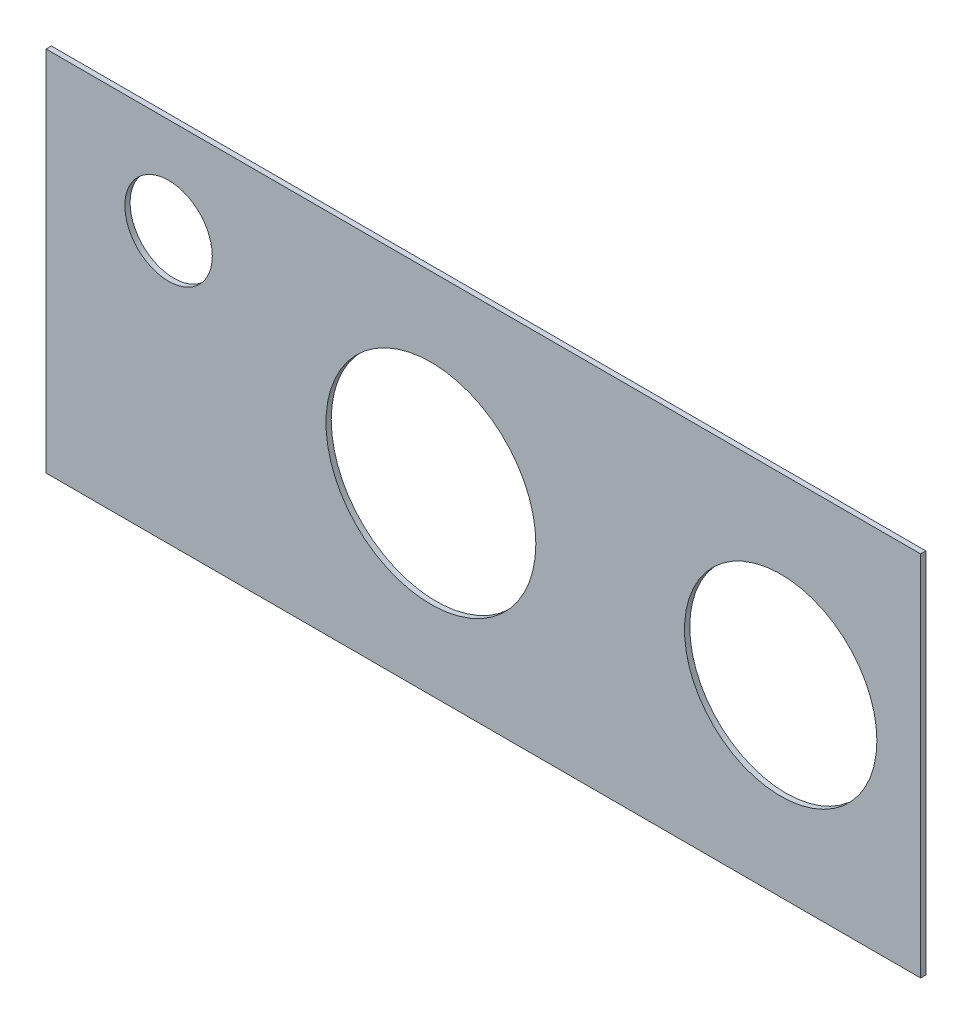
SolidWorks part; units mm, degrees
ref_plane "Front Plane" through (0, 0, 0) normal (0, 0, 1) x (1, 0, 0)
ref_plane "Top Plane" through (0, 0, 0) normal (0, 1, 0) x (1, 0, 0)
ref_plane "Right Plane" through (0, 0, 0) normal (1, 0, 0) x (0, 0, -1)
sketch "Sketch1" plane through (0, 0, 0) normal (0, 0, 1) x (1, 0, 0)
  line L1 (0, 0) -> (500, 0)
  line L2 (0, 0) -> (0, 210)
  line L3 (0, 210) -> (500, 210)
  line L4 (500, 0) -> (500, 210)
  dimension "D1" = 500
  dimension "D2" = 210
extrude "Boss-Extrude1" add sketch "Sketch1" along normal blind 3
extrude "Cut-Extrude1" cut sketch "Sketch2" against normal blind 10
sketch "Sketch2" plane through (492, 10, 3) normal (0, 0, 1) x (1, 0, 0)
  circle A0 centre (-72, 95) radius 55
  circle A1 centre (-272, 95) radius 60
  circle A2 centre (-422, 145) radius 25
